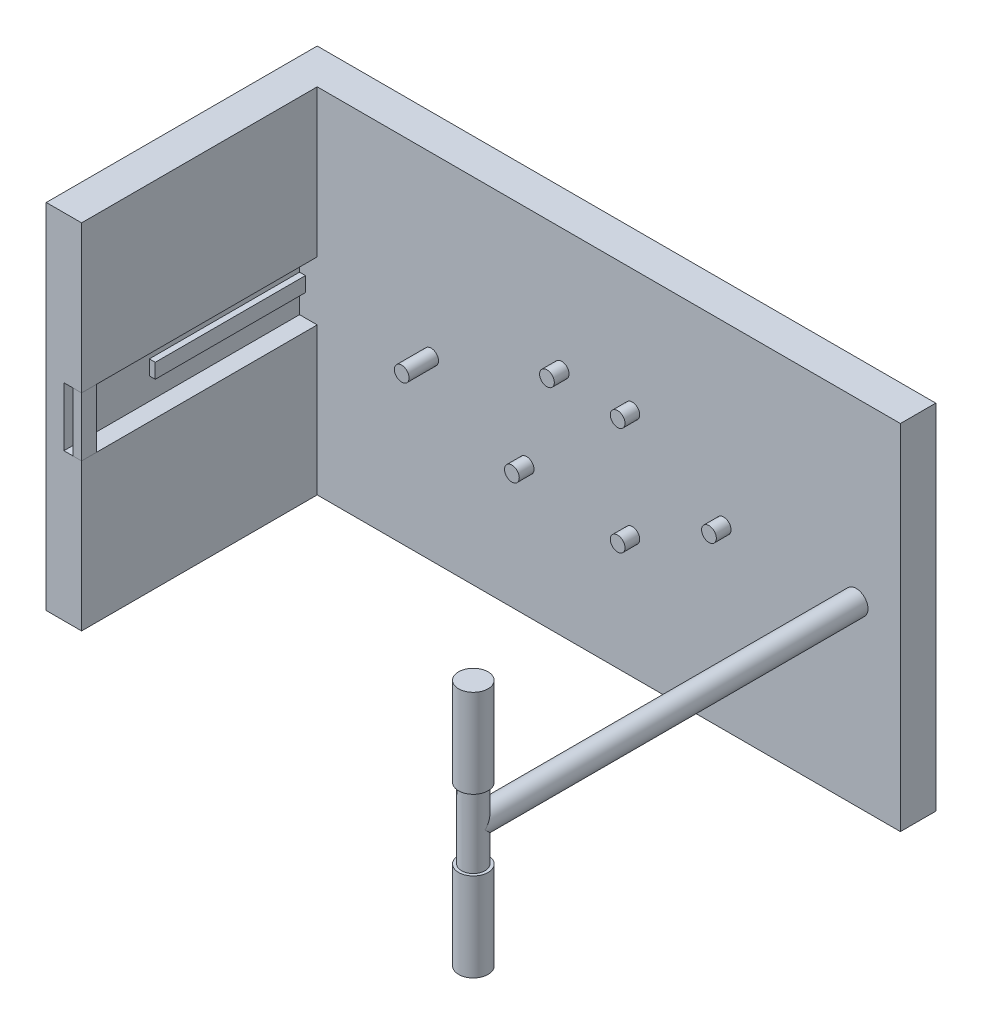
from build123d import *

# Parameters (mm, degrees)
SKETCH2_W                = 2100
SKETCH2_H                = 1200
BOSS_EXTRUDE1_DEPTH      = 120
SKETCH3_W                = 120
SKETCH3_H                = 1200
BOSS_EXTRUDE2_DEPTH      = 800
SKETCH4_R                = 40
BOSS_EXTRUDE3_DEPTH      = 1300
BOSS_EXTRUDE4_DEPTH      = 120
BOSS_EXTRUDE4_DEPTH_BACK = 120
SKETCH6_R                = 40
BOSS_EXTRUDE5_START      = 120
SKETCH7_R                = 50
BOSS_EXTRUDE5_DEPTH      = 300
SKETCH9_R                = 25
BOSS_EXTRUDE6_DEPTH      = 50
SKETCH10_R               = 25
BOSS_EXTRUDE7_DEPTH      = 50
SKETCH11_R               = 25
BOSS_EXTRUDE8_DEPTH      = 50
SKETCH12_R               = 25
BOSS_EXTRUDE9_DEPTH      = 50
SKETCH13_R               = 25
BOSS_EXTRUDE10_DEPTH     = 100
SKETCH14_W               = 120
SKETCH14_H               = 200
CUT_EXTRUDE1_DEPTH       = 800
SKETCH15_W               = 510
SKETCH15_H               = 50
BOSS_EXTRUDE11_DEPTH     = 20
SKETCH16_W               = 30
SKETCH16_H               = 50
BOSS_EXTRUDE12_DEPTH     = 200


with BuildPart() as part:
    # Sketch2 → Boss-Extrude1 (new body)
    with BuildSketch(Plane.XY):
        with Locations((1050, -600)):
            Rectangle(SKETCH2_W, SKETCH2_H)
    extrude(amount=BOSS_EXTRUDE1_DEPTH)

    # Sketch3 → Boss-Extrude2 (add)
    with BuildSketch(Plane.XY.offset(120)):
        with Locations((60, -600)):
            Rectangle(SKETCH3_W, SKETCH3_H)
    extrude(amount=BOSS_EXTRUDE2_DEPTH)

    # Sketch4 → Boss-Extrude3 (add)
    with BuildSketch(Plane.XY.offset(120)):
        with Locations((1950, -600)):
            Circle(SKETCH4_R)
    extrude(amount=BOSS_EXTRUDE3_DEPTH)

    # Sketch6 → Boss-Extrude4 (add, two sides: drawn at the far end of the back side and taken through both)
    with BuildSketch(Plane(origin=(0, -600, 0), x_dir=(-1, 0, 0), z_dir=(0, -1, 0)).offset(-BOSS_EXTRUDE4_DEPTH_BACK)):
        with Locations(Location((-1950, -1420, 0), (0, 0, 90))):
            Circle(SKETCH6_R)
    extrude(amount=BOSS_EXTRUDE4_DEPTH + BOSS_EXTRUDE4_DEPTH_BACK)

    # Sketch7 → Boss-Extrude5 (add)
    with BuildSketch(Plane(origin=(0, -600, 0), x_dir=(-1, 0, 0), z_dir=(0, -1, 0)).offset(BOSS_EXTRUDE5_START)):
        with Locations(Location((-1950, -1420, 0), (0, 0, 90))):
            Circle(SKETCH7_R)
    boss_extrude5 = extrude(amount=BOSS_EXTRUDE5_DEPTH)

    # Mirror1: Boss-Extrude5 across plane
    add(boss_extrude5.mirror(Plane(origin=(0, -600, 0), x_dir=(0, 0, 1), z_dir=(0, -1, 0))))

    # Sketch9 → Boss-Extrude6 (add)
    with BuildSketch(Plane.XY.offset(120)):
        with Locations((1500, -600)):
            Circle(SKETCH9_R)
    extrude(amount=BOSS_EXTRUDE6_DEPTH)

    # Sketch10 → Boss-Extrude7 (add)
    with BuildSketch(Plane.XY.offset(120)):
        with Locations((1190, -416.969947823)):
            Circle(SKETCH10_R)
        with Locations((1190, -783.030052177)):
            Circle(SKETCH10_R)
    extrude(amount=BOSS_EXTRUDE7_DEPTH)

    # Sketch11 → Boss-Extrude8 (add)
    with BuildSketch(Plane.XY.offset(120)):
        with Locations((950, -416.969947823)):
            Circle(SKETCH11_R)
    extrude(amount=BOSS_EXTRUDE8_DEPTH)

    # Sketch12 → Boss-Extrude9 (add)
    with BuildSketch(Plane.XY.offset(120)):
        with Locations((830.962699777, -756.720034145)):
            Circle(SKETCH12_R)
    extrude(amount=BOSS_EXTRUDE9_DEPTH)

    # Sketch13 → Boss-Extrude10 (add)
    with BuildSketch(Plane.XY.offset(120)):
        with Locations((506.86575302, -600)):
            Circle(SKETCH13_R)
    extrude(amount=BOSS_EXTRUDE10_DEPTH)

    # Sketch14 → Cut-Extrude1 (cut)
    with BuildSketch(Plane.XY.offset(920)):
        with Locations((120, -600)):
            Rectangle(SKETCH14_W, SKETCH14_H)
    extrude(amount=-CUT_EXTRUDE1_DEPTH, mode=Mode.SUBTRACT)

    # Sketch15 → Boss-Extrude11 (add)
    with BuildSketch(Plane(origin=(60, 0, 0), x_dir=(0, 0, -1), z_dir=(1, 0, 0))):
        with Locations((-375, -600)):
            Rectangle(SKETCH15_W, SKETCH15_H)
    extrude(amount=BOSS_EXTRUDE11_DEPTH)


with BuildPart() as body_2:
    # Sketch16 → Boss-Extrude12 (new body)
    with BuildSketch(Plane.XZ.offset(500)):
        with Locations((105, 895)):
            Rectangle(SKETCH16_W, SKETCH16_H)
    extrude(amount=BOSS_EXTRUDE12_DEPTH)


solid = Compound([part.part, body_2.part])
